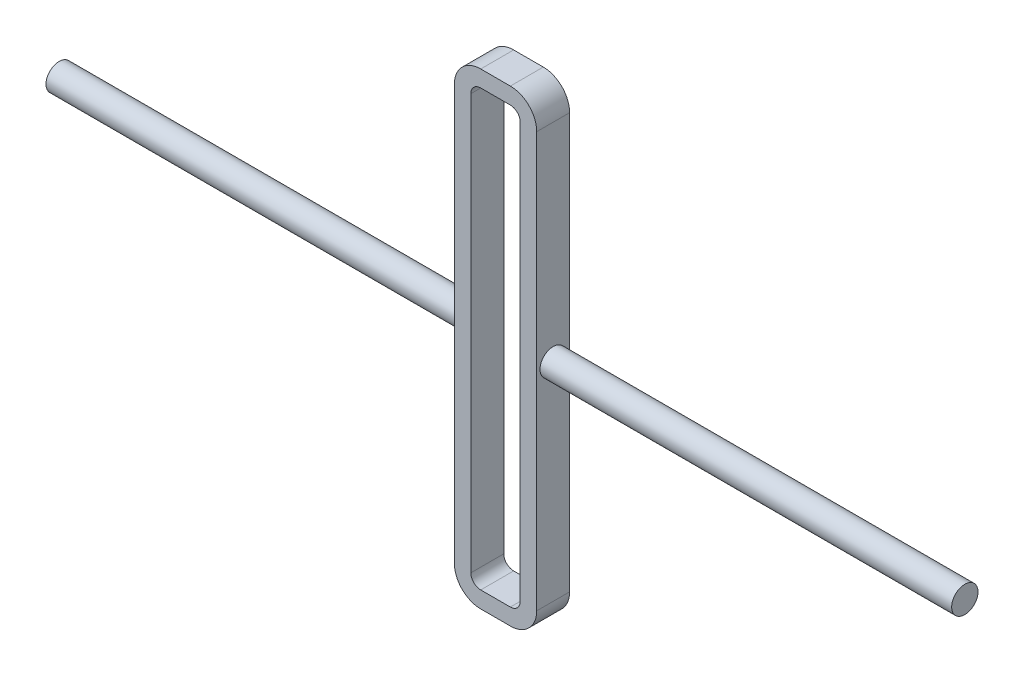
from build123d import *

# Parameters (mm, degrees)
BOSS_EXTRUDE1_DEPTH = 10
SKETCH2_R           = 4
BOSS_EXTRUDE2_DEPTH = 125
BOSS_EXTRUDE3_START = 125
SKETCH3_R           = 4
BOSS_EXTRUDE3_DEPTH = 125


with BuildPart() as part:
    # Sketch1 → Boss-Extrude1 (new body)
    with BuildSketch(Plane.XY):
        with BuildLine():
            Line((-4.5, 71), (4.5, 71))
            ThreePointArc((4.5, 71), (10.156854249, 68.656854249), (12.5, 63))
            Line((12.5, 63), (12.5, -63))
            ThreePointArc((12.5, -63), (10.156854249, -68.656854249), (4.5, -71))
            Line((4.5, -71), (-4.5, -71))
            ThreePointArc((-4.5, -71), (-10.156854249, -68.656854249), (-12.5, -63))
            Line((-12.5, -63), (-12.5, 63))
            ThreePointArc((-12.5, 63), (-10.156854249, 68.656854249), (-4.5, 71))
        make_face()
        with BuildLine():
            Line((-4.5, 66), (4.5, 66))
            ThreePointArc((4.5, 66), (6.621320344, 65.121320344), (7.5, 63))
            Line((7.5, 63), (7.5, -63))
            ThreePointArc((7.5, -63), (6.621320344, -65.121320344), (4.5, -66))
            Line((4.5, -66), (-4.5, -66))
            ThreePointArc((-4.5, -66), (-6.621320344, -65.121320344), (-7.5, -63))
            Line((-7.5, -63), (-7.5, 63))
            ThreePointArc((-7.5, 63), (-6.621320344, 65.121320344), (-4.5, 66))
        make_face(mode=Mode.SUBTRACT)
    extrude(amount=BOSS_EXTRUDE1_DEPTH)

    # Sketch2 → Boss-Extrude2 (add)
    with BuildSketch(Plane(origin=(12.5, 0, 0), x_dir=(0, 0, -1), z_dir=(1, 0, 0))):
        with Locations(Location((-5, 0, 0), (0, 0, 270))):
            Circle(SKETCH2_R)
    extrude(amount=BOSS_EXTRUDE2_DEPTH)

    # Sketch3 → Boss-Extrude3 (add)
    with BuildSketch(Plane.ZY.offset(12.5).offset(BOSS_EXTRUDE3_START)):
        with Locations(Location((5, 0, 0), (0, 0, 270))):
            Circle(SKETCH3_R)
    extrude(amount=-BOSS_EXTRUDE3_DEPTH)


solid = part.part
